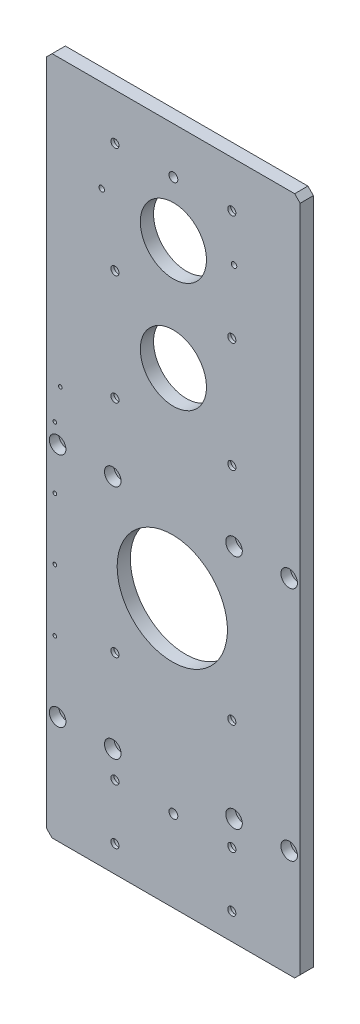
from build123d import *

# Parameters (mm, degrees)
SKETCH_1_W                   = 230
SKETCH_1_H                   = 616
EXTRUDE_1_DEPTH              = 12
CHAMFER_1_SIZE               = 5
HOLE_WIZARD_M8_1_D           = 9
HOLE_WIZARD_M8_1_DEPTH       = 11.5
HOLE_WIZARD_M8_1_CBORE_D     = 15
HOLE_WIZARD_M8_1_CBORE_DEPTH = 8.6
HOLE_WIZARD_M8_1_TIP         = 2.703872786
HOLE_WIZARD_M8_2_D           = 9
HOLE_WIZARD_M8_2_DEPTH       = 22.25
HOLE_WIZARD_M8_2_CBORE_D     = 15
HOLE_WIZARD_M8_2_CBORE_DEPTH = 8.6
HOLE_WIZARD_M8_2_TIP         = 2.703872786
MM_1_D                       = 8
MM_1_DEPTH                   = 22.25
MM_1_TIP                     = 2.403442476
HOLE_WIZARD_M4_1_D           = 3.3
HOLE_WIZARD_M4_2_D           = 3.3
SKETCH_12_R                  = 30
SKETCH_12_R_2                = 50
CUT_EXTRUDE_1_DEPTH          = 665.059688056
HOLE_WIZARD_M6_1_D           = 5
HOLE_WIZARD_M6_1_DEPTH       = 17
HOLE_WIZARD_M6_1_TIP         = 1.502151548


with BuildPart() as part:
    # 草图1 → 凸台-拉伸1 (new body)
    with BuildSketch(Plane.XY):
        with Locations((95.026115454, 321.857364907)):
            Rectangle(SKETCH_1_W, SKETCH_1_H)
    extrude(amount=EXTRUDE_1_DEPTH)

    # 倒角1
    chamfer_1_edges = [part.edges().sort_by_distance(p)[0] for p in [
        (210.026115454, 13.857364907, 6),
        (-19.973884546, 13.857364907, 6),
        (-19.973884546, 629.857364907, 6),
        (210.026115454, 629.857364907, 6),
    ]]
    chamfer(chamfer_1_edges, length=CHAMFER_1_SIZE)

    # M8 六角凹头螺钉的柱形沉头孔1
    with Locations(Plane(origin=(0, 0, 0), x_dir=(-1, 0, 0), z_dir=(0, 0, -1))):
        with Locations((-148.026115454, 587.857364907), (-42.026115454, 587.857364907), (-148.026115454, 487.857364907), (-42.026115454, 487.857364907), (-148.026115454, 387.857364907), (-42.026115454, 387.857364907), (-148.026115454, 187.857364907), (-42.026115454, 187.857364907), (-148.026115454, 87.857364907), (-42.026115454, 87.857364907), (-148.026115454, 37.857364907), (-42.026115454, 37.857364907)):
            CounterBoreHole(HOLE_WIZARD_M8_1_D / 2, HOLE_WIZARD_M8_1_CBORE_D / 2, HOLE_WIZARD_M8_1_CBORE_DEPTH, depth=HOLE_WIZARD_M8_1_DEPTH)
            with Locations((0, 0, -(HOLE_WIZARD_M8_1_DEPTH + HOLE_WIZARD_M8_1_TIP / 2))):  # 118° drill point
                Cone(0, HOLE_WIZARD_M8_1_D / 2, HOLE_WIZARD_M8_1_TIP, mode=Mode.SUBTRACT)

    # M8 六角凹头螺钉的柱形沉头孔2
    with Locations(Plane.XY.offset(12)):
        with Locations((-9.973884546, 325.357364907), (40.026115454, 325.357364907), (150.026115454, 325.357364907), (200.026115454, 325.357364907), (-9.973884546, 111.357364907), (40.026115454, 111.357364907), (150.026115454, 111.357364907), (200.026115454, 111.357364907)):
            CounterBoreHole(HOLE_WIZARD_M8_2_D / 2, HOLE_WIZARD_M8_2_CBORE_D / 2, HOLE_WIZARD_M8_2_CBORE_DEPTH, depth=HOLE_WIZARD_M8_2_DEPTH)
            with Locations((0, 0, -(HOLE_WIZARD_M8_2_DEPTH + HOLE_WIZARD_M8_2_TIP / 2))):  # 118° drill point
                Cone(0, HOLE_WIZARD_M8_2_D / 2, HOLE_WIZARD_M8_2_TIP, mode=Mode.SUBTRACT)

    # 大小mm 暗销孔1
    with Locations(Plane.XY.offset(12)):
        with Locations((95.026115454, 587.857364907), (95.026115454, 87.857364907)):
            Hole(MM_1_D / 2, depth=MM_1_DEPTH)
            with Locations((0, 0, -(MM_1_DEPTH + MM_1_TIP / 2))):  # 118° drill point
                Cone(0, MM_1_D / 2, MM_1_TIP, mode=Mode.SUBTRACT)

    # M4 螺纹孔1 (through all)
    with Locations(Plane.XY.offset(12)):
        with Locations((-12.473884546, 341.857364907), (-12.473884546, 285.857364907), (-12.473884546, 229.857364907), (-12.473884546, 173.857364907)):
            Hole(HOLE_WIZARD_M4_1_D / 2)

    # M4 螺纹孔2 (through all)
    with Locations(Plane.XY.offset(12)):
        with Locations((-7.473884546, 371.857364907)):
            Hole(HOLE_WIZARD_M4_2_D / 2)

    # 草图12 → 切除-拉伸1 (cut, through all)
    with BuildSketch(Plane(origin=(0, 0, 0), x_dir=(-1, 0, 0), z_dir=(0, 0, -1))):
        with Locations((-95.026115454, 537.857364907)):
            Circle(SKETCH_12_R)
        with Locations((-95.026115454, 437.857364907)):
            Circle(SKETCH_12_R)
        with Locations((-94.026115454, 256.607364907)):
            Circle(SKETCH_12_R_2)
    extrude(amount=-CUT_EXTRUDE_1_DEPTH, mode=Mode.SUBTRACT)

    # M6 螺纹孔1
    with Locations(Plane(origin=(0, 0, 0), x_dir=(-1, 0, 0), z_dir=(0, 0, -1))):
        with Locations((-150.026115454, 546.357364907), (-30.026115454, 546.357364907)):
            Hole(HOLE_WIZARD_M6_1_D / 2, depth=HOLE_WIZARD_M6_1_DEPTH)
            with Locations((0, 0, -(HOLE_WIZARD_M6_1_DEPTH + HOLE_WIZARD_M6_1_TIP / 2))):  # 118° drill point
                Cone(0, HOLE_WIZARD_M6_1_D / 2, HOLE_WIZARD_M6_1_TIP, mode=Mode.SUBTRACT)


solid = part.part
